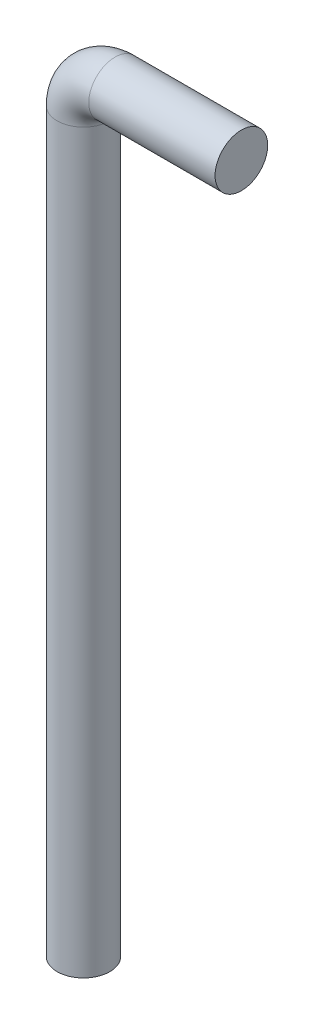
from build123d import *

# Parameters (mm, degrees)
SKETCH_16_R = 2.5


with BuildPart() as part:
    # 扫描1: sweep along a path in 草图17
    with BuildLine(Plane.XY) as sweep_1_path:
        Line((0, 0), (0, 70))
        ThreePointArc((0, 70), (0.878679656, 72.121320344), (3, 73))
        Line((3, 73), (15, 73))
    # 草图16 → 扫描1 (sweep)
    with BuildSketch(Plane(origin=(0, 0, 0), x_dir=(1, 0, 0), z_dir=(0, 1, 0))):
        Circle(SKETCH_16_R)
    sweep(path=sweep_1_path.line)


solid = part.part
